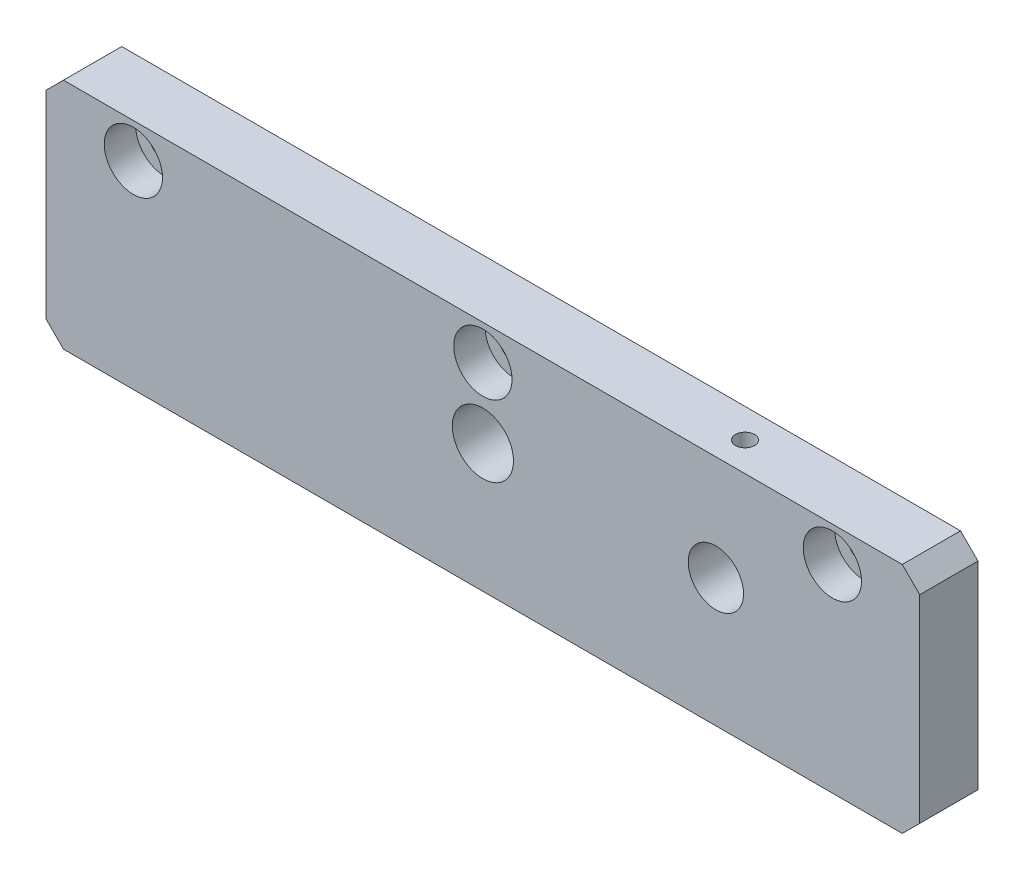
SolidWorks part; units mm, degrees
material "6061"
ref_plane "Front Plane" through (0, 0, 0) normal (0, 0, 1) x (1, 0, 0)
ref_plane "Top Plane" through (0, 0, 0) normal (0, 1, 0) x (1, 0, 0)
ref_plane "Right Plane" through (0, 0, 0) normal (1, 0, 0) x (0, 0, -1)
sketch "Sketch1" plane through (0, 0, 0) normal (0, 0, 1) x (1, 0, 0)
  line L1 (-75, 20) -> (75, 20)
  line L2 (-75, 20) -> (-75, -20)
  line L3 (-75, -20) -> (75, -20)
  line L4 (75, 20) -> (75, -20)
  line L5 (-75, 20) -> (75, -20) construction
  line L6 (-75, -20) -> (75, 20) construction
  point P0 (0, 0)
  dimension "D1" = 150
  dimension "D2" = 40
extrude "Boss-Extrude1" add sketch "Sketch1" along normal blind 10
sketch "Sketch2" plane through (0, 0, 10) normal (0, 0, 1) x (1, 0, 0)
  line L0 (-75, -20) -> (75, -20) construction
  line L1 (0, 0) -> (0, 20) construction
  line L2 (75, 20) -> (-75, 20) construction
  circle A0 centre (40, 2) radius 4.75
  dimension "D1" = 22
  dimension "D3" = 9.5
  dimension "D2" = 40
extrude "Cut-Extrude1" cut sketch "Sketch2" against normal through all
hole_wizard "Ø10.5 (10.5) Diameter Hole1" positions "Sketch4" profile "Sketch3" hole size "Ø10.5" standard "Iso"
sketch "Sketch4" plane through (0, 0, 10) normal (0, 0, 1) x (1, 0, 0)
  line L0 (0, 0) -> (0, -20) construction
  line L1 (-75, -20) -> (75, -20) construction
  point P0 (0, 2)
  dimension "D1" = 22
sketch "Sketch3" plane through (0, 2, 10) normal (1, 0, 0) x (0, -1, 0)
  line L0 (0, 0) -> (0, 79.1545)
  line L1 (0, 79.1545) -> (5.25, 76)
  line L2 (5.25, 76) -> (5.25, 0)
  line L5 (5.25, 0) -> (0, 0)
  line L10 (0, 79.1545) -> (-5.25, 76) construction
  line L11 (0, -6.35) -> (0, 107.95) construction
  dimension "孔直径" = 10.5
  dimension "孔深度" = 76
  dimension "导头角度" = 118
hole_wizard "CBORE for M5 Hex Socket Head Cap Screw1" positions "Sketch6" profile "Sketch5" counterbore size "M5" standard "Iso" end condition through all
sketch "Sketch6" plane through (0, 0, 10) normal (0, 0, 1) x (1, 0, 0)
  line L0 (0, 0) -> (0, -20) construction
  line L1 (-75, -20) -> (75, -20) construction
  line L3 (75, 20) -> (-75, 20) construction
  point P0 (60, 14)
  point P2 (0, 14)
  point P4 (-60, 14)
  dimension "D1" = 6
  dimension "D2" = 120
sketch "Sketch5" plane through (60, 14, 10) normal (1, 0, 0) x (0, -1, 0)
  line L0 (0, 0) -> (0, 10)
  line L1 (0, 10) -> (2.75, 10)
  line L3 (2.75, 10) -> (2.75, 5.4)
  line L4 (2.75, 5.4) -> (5, 5.4)
  line L5 (5, 5.4) -> (5, 0)
  line L7 (5, 0) -> (0, 0)
  line L11 (0, -6.35) -> (0, 107.95) construction
  dimension "通孔孔直径" = 5.5
  dimension "通孔孔深度" = 10
  dimension "柱形沉头孔直径" = 10
  dimension "柱形沉头孔深度" = 5.4
hole_wizard "M4 Tapped Hole1" positions "Sketch8" profile "Sketch7" tap size "M4" standard "Iso"
sketch "Sketch8" plane through (0, 20, 0) normal (0, 1, 0) x (1, 0, 0)
  line L0 (40, -10) -> (40, 0) construction
  line L1 (75, -10) -> (-75, -10) construction
  line L2 (75, 0) -> (-75, 0) construction
  point P0 (40, -5)
  point P10 (0, 0)
  dimension "D1" = 40
cosmetic thread "Hole thread1" parameters "D2"=4
sketch "Sketch7" plane through (40, 20, 5) normal (1, 0, 0) x (0, 0, 1)
  line L0 (0, 0) -> (0, 13.25)
  line L1 (0, 13.25) -> (1.65, 13.25)
  line L2 (1.65, 13.25) -> (1.65, 0)
  line L5 (1.65, 0) -> (0, 0)
  line L11 (0, -6.35) -> (0, 107.95) construction
  dimension "通孔螺纹孔钻头直径" = 3.3
  dimension "通孔螺纹孔钻头深度" = 13.25
chamfer "Chamfer1" distance 3 angle 45 4 edges at (75, -20, 5) (-75, -20, 5) (-75, 20, 5) (75, 20, 5)
